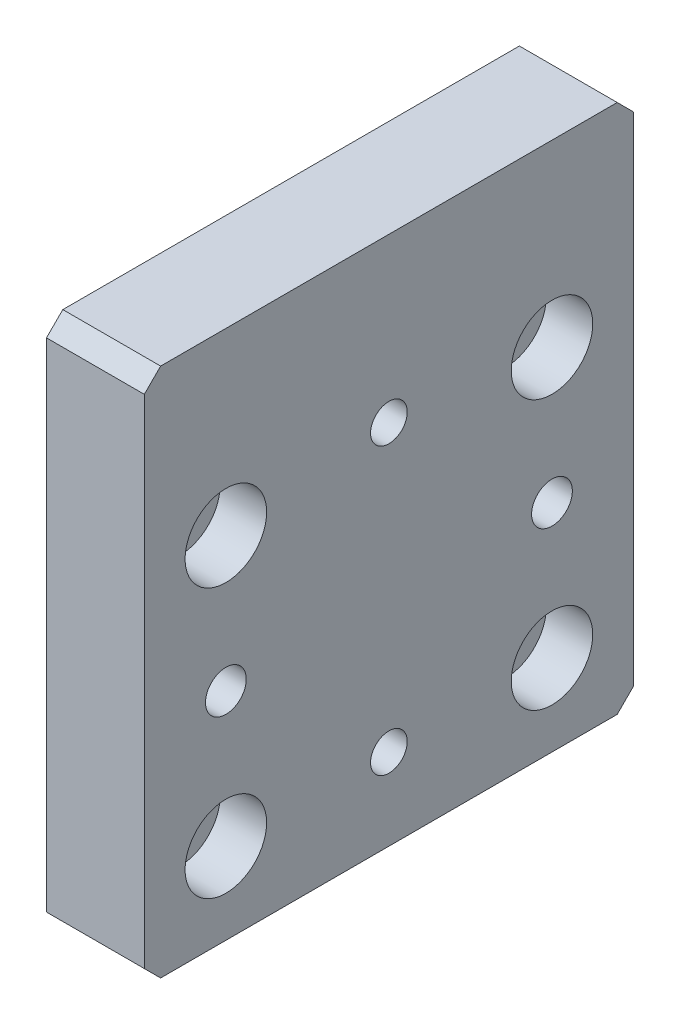
from build123d import *

# Parameters (mm, degrees)
SKETCH1_W                                            = 60
SKETCH1_H                                            = 65
BOSS_EXTRUDE1_DEPTH                                  = 12
CBORE_FOR_M4_HEXAGON_SOCKET_HEAD_CAP_SCR_D           = 4.5
CBORE_FOR_M4_HEXAGON_SOCKET_HEAD_CAP_SCR_CBORE_D     = 8
CBORE_FOR_M4_HEXAGON_SOCKET_HEAD_CAP_SCR_CBORE_DEPTH = 4.6
CBORE_FOR_M5_HEXAGON_SOCKET_HEAD_CAP_SCR_D           = 5.5
CBORE_FOR_M5_HEXAGON_SOCKET_HEAD_CAP_SCR_CBORE_D     = 10
CBORE_FOR_M5_HEXAGON_SOCKET_HEAD_CAP_SCR_CBORE_DEPTH = 5.7
CHAMFER1_SIZE                                        = 2
F_5_0MM_BLIND_DOWEL_HOLE1_D                          = 5


with BuildPart() as part:
    # Sketch1 → Boss-Extrude1 (new body)
    with BuildSketch(Plane(origin=(0, 0, 0), x_dir=(0, 0, -1), z_dir=(1, 0, 0))):
        Rectangle(SKETCH1_W, SKETCH1_H)
    extrude(amount=BOSS_EXTRUDE1_DEPTH)

    # CBORE for M4 Hexagon socket head cap screws1 (through all)
    with Locations(Plane.ZY):
        with Locations((0, 12.5), (0, -22.5)):
            CounterBoreHole(CBORE_FOR_M4_HEXAGON_SOCKET_HEAD_CAP_SCR_D / 2, CBORE_FOR_M4_HEXAGON_SOCKET_HEAD_CAP_SCR_CBORE_D / 2, CBORE_FOR_M4_HEXAGON_SOCKET_HEAD_CAP_SCR_CBORE_DEPTH)

    # CBORE for M5 Hexagon socket head cap screws1 (through all)
    with Locations(Plane(origin=(12, 0, 0), x_dir=(0, 0, -1), z_dir=(1, 0, 0))):
        with Locations((-20, 10.5), (-20, -22.5), (20, -22.5), (20, 10.5)):
            CounterBoreHole(CBORE_FOR_M5_HEXAGON_SOCKET_HEAD_CAP_SCR_D / 2, CBORE_FOR_M5_HEXAGON_SOCKET_HEAD_CAP_SCR_CBORE_D / 2, CBORE_FOR_M5_HEXAGON_SOCKET_HEAD_CAP_SCR_CBORE_DEPTH)

    # Chamfer1
    chamfer1_edges = [part.edges().sort_by_distance(p)[0] for p in [
        (6, -32.5, -30),
        (6, -32.5, 30),
        (6, 32.5, 30),
        (6, 32.5, -30),
    ]]
    chamfer(chamfer1_edges, length=CHAMFER1_SIZE)

    # Ø5.0mm blind dowel hole1 (through all)
    with Locations(Plane(origin=(12, 0, 0), x_dir=(0, 0, -1), z_dir=(1, 0, 0))):
        with Locations((-20, -6), (20, -6)):
            Hole(F_5_0MM_BLIND_DOWEL_HOLE1_D / 2)


solid = part.part
